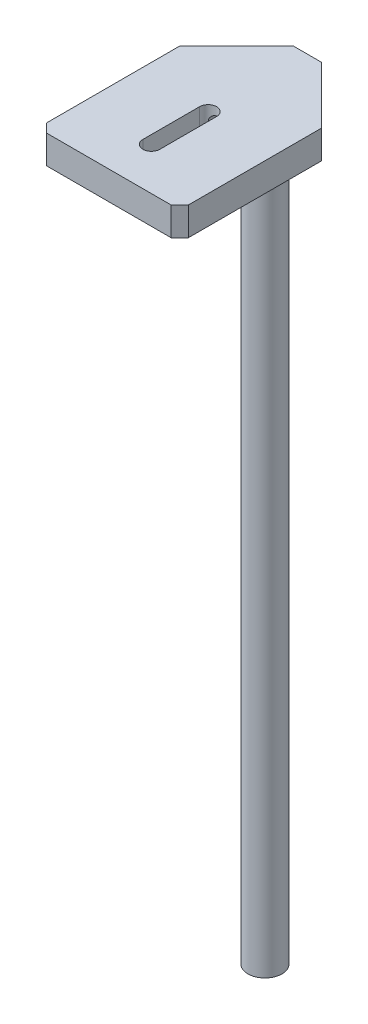
from build123d import *

# Parameters (mm, degrees)
BOSS_EXTRUDE1_DEPTH   = 10
SKETCH2_R             = 6
BOSS_EXTRUDE2_DEPTH   = 260
M5_TAPPED_HOLE1_D     = 4.2
M5_TAPPED_HOLE1_DEPTH = 36.9
M5_TAPPED_HOLE1_TIP   = 1.2618073
CUT_EXTRUDE1_DEPTH    = 266.047165614
CHAMFER1_SIZE         = 3


with BuildPart() as part:
    # Sketch1 → Boss-Extrude1 (new body)
    with BuildSketch(Plane(origin=(0, 0, 0), x_dir=(1, 0, 0), z_dir=(0, 1, 0))):
        Polygon((-25, 25), (-5, 45), (5, 45), (25, 25), (25, -25), (-25, -25), align=None)
    extrude(amount=BOSS_EXTRUDE1_DEPTH)

    # Sketch2 → Boss-Extrude2 (add)
    with BuildSketch(Plane.XZ):
        with Locations(Location((0, -30, 0), (0, 0, 90))):
            Circle(SKETCH2_R)
    extrude(amount=BOSS_EXTRUDE2_DEPTH)

    # M5 Tapped Hole1
    with Locations(Plane(origin=(0, 0, -45), x_dir=(-1, 0, 0), z_dir=(0, 0, -1))):
        with Locations((0, 5)):
            Hole(M5_TAPPED_HOLE1_D / 2, depth=M5_TAPPED_HOLE1_DEPTH)
            with Locations((0, 0, -(M5_TAPPED_HOLE1_DEPTH + M5_TAPPED_HOLE1_TIP / 2))):  # 118° drill point
                Cone(0, M5_TAPPED_HOLE1_D / 2, M5_TAPPED_HOLE1_TIP, mode=Mode.SUBTRACT)

    # Sketch5 → Cut-Extrude1 (cut, through all)
    with BuildSketch(Plane.XZ):
        with BuildLine():
            Line((3, 10), (3, -10))
            ThreePointArc((3, -10), (0, -13), (-3, -10))
            Line((-3, -10), (-3, 10))
            ThreePointArc((-3, 10), (0, 13), (3, 10))
        make_face()
    extrude(amount=-CUT_EXTRUDE1_DEPTH, mode=Mode.SUBTRACT)

    # Chamfer1
    chamfer1_edges = [part.edges().sort_by_distance(p)[0] for p in [
        (25, 5, 25),
        (-25, 5, 25),
    ]]
    chamfer(chamfer1_edges, length=CHAMFER1_SIZE)


solid = part.part
